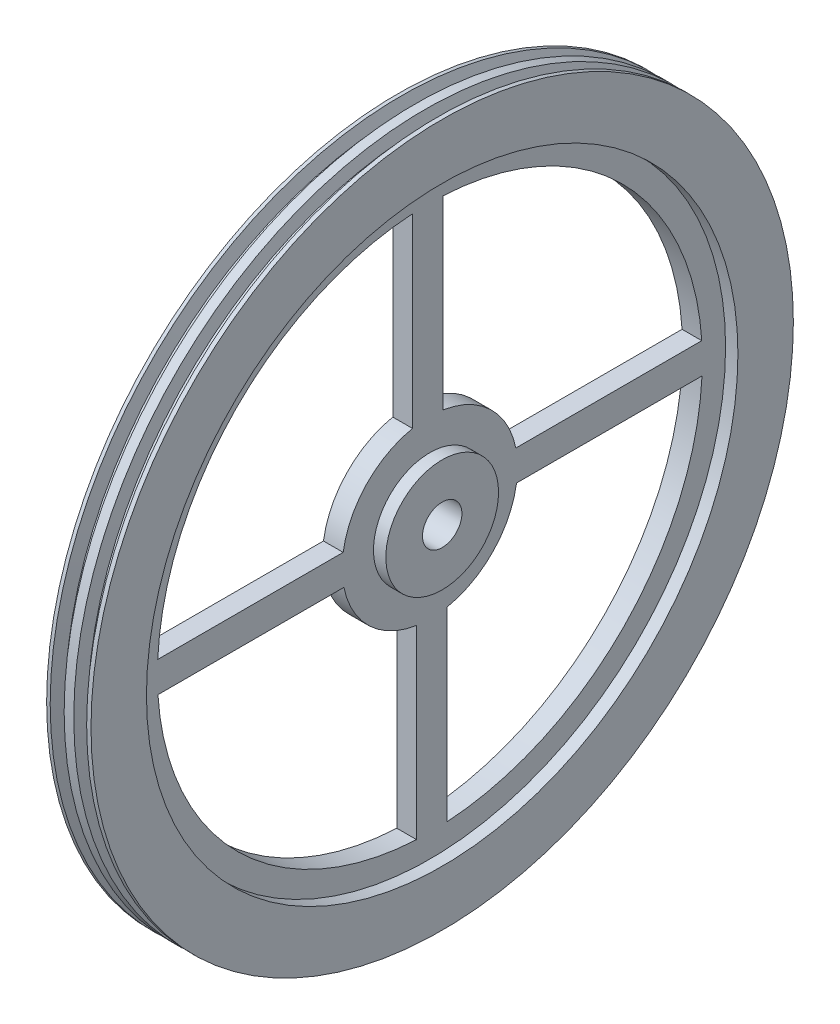
from build123d import *

# Parameters (mm, degrees)
SKETCH2_R           = 120
CUT_EXTRUDE1_DEPTH  = 5
CUT_EXTRUDE2_START  = -5
SKETCH3_R           = 120
CUT_EXTRUDE2_DEPTH  = 5
SKETCH4_R           = 8
CUT_EXTRUDE3_DEPTH  = 202.944299251
BOSS_EXTRUDE1_START = 5
SKETCH5_R           = 22.870444207
SKETCH5_R_2         = 8
BOSS_EXTRUDE1_DEPTH = 5
SKETCH6_R           = 22.870444207
SKETCH6_R_2         = 8
BOSS_EXTRUDE2_DEPTH = 5
CUT_EXTRUDE5_DEPTH  = 202.944299251
CIRPATTERN1_COUNT   = 4


with BuildPart() as part:
    # Sketch1 → Revolve1 (revolve)
    with BuildSketch(Plane(origin=(0, 0, 0), x_dir=(1, 0, 0), z_dir=(0, 1, 0)), mode=Mode.PRIVATE) as revolve1_sk:
        Polygon((0, 0), (0, 142.5), (1.439897502, 142.5), (3.207174134, 138.107099477), (5.784452556, 138.107099477), (7.10991003, 142.5), (11.012645925, 142.5), (12.264466873, 138.107099477), (14.915381821, 138.107099477), (16.240839295, 142.5), (18, 142.5), (18, 0), align=None)
    revolve(revolve1_sk.sketch.rotate(Axis((0, 0, 0), (1, 0, 0)), 180), axis=Axis((0, 0, 0), (1, 0, 0)))

    # Sketch2 → Cut-Extrude1 (cut)
    with BuildSketch(Plane.ZY):
        Circle(SKETCH2_R)
    extrude(amount=-CUT_EXTRUDE1_DEPTH, mode=Mode.SUBTRACT)

    # Sketch3 → Cut-Extrude2 (cut)
    with BuildSketch(Plane(origin=(18, 0, 0), x_dir=(0, 0, -1), z_dir=(1, 0, 0)).offset(CUT_EXTRUDE2_START)):
        with Locations(Location((0, 0, 0), (0, 0, 180))):
            Circle(SKETCH3_R)
    extrude(amount=CUT_EXTRUDE2_DEPTH, mode=Mode.SUBTRACT)

    # Sketch4 → Cut-Extrude3 (cut, through all)
    with BuildSketch(Plane(origin=(13, 0, 0), x_dir=(0, 0, -1), z_dir=(1, 0, 0))):
        Circle(SKETCH4_R)
    extrude(amount=-CUT_EXTRUDE3_DEPTH, mode=Mode.SUBTRACT)

    # Sketch5 → Boss-Extrude1 (add)
    with BuildSketch(Plane(origin=(13, 0, 0), x_dir=(0, 0, -1), z_dir=(1, 0, 0)).offset(BOSS_EXTRUDE1_START)):
        Circle(SKETCH5_R)
        Circle(SKETCH5_R_2, mode=Mode.SUBTRACT)
    extrude(amount=-BOSS_EXTRUDE1_DEPTH)

    # Sketch6 → Boss-Extrude2 (add)
    with BuildSketch(Plane.ZY.offset(-5)):
        with Locations(Location((0, 0, 0), (0, 0, 180))):
            Circle(SKETCH6_R)
        with Locations(Location((0, 0, 0), (0, 0, 180))):
            Circle(SKETCH6_R_2, mode=Mode.SUBTRACT)
    extrude(amount=BOSS_EXTRUDE2_DEPTH)

    # Sketch7 → Cut-Extrude5 (cut, through all)
    with BuildSketch(Plane.ZY.offset(-5)):
        with BuildLine():
            Line((-5.40203869, 35.175568579), (-5.40203869, 110.423122323))
            ThreePointArc((-5.40203869, 110.423122323), (-77.592767083, 78.751574346), (-110.330916303, 7.038243628))
            Line((-110.330916303, 7.038243628), (-34.885036528, 7.038243628))
            ThreePointArc((-34.885036528, 7.038243628), (-24.57009099, 25.745160237), (-5.40203869, 35.175568579))
        make_face()
    cut_extrude5 = extrude(amount=-CUT_EXTRUDE5_DEPTH, mode=Mode.SUBTRACT)

    # CirPattern1: Cut-Extrude5 ×4 about axis
    cirpattern1_axis = Axis((0, 0, 0), (1, 0, 0))
    for i in range(1, CIRPATTERN1_COUNT):
        add(cut_extrude5.rotate(cirpattern1_axis, i * 360 / CIRPATTERN1_COUNT), mode=Mode.SUBTRACT)


solid = part.part
